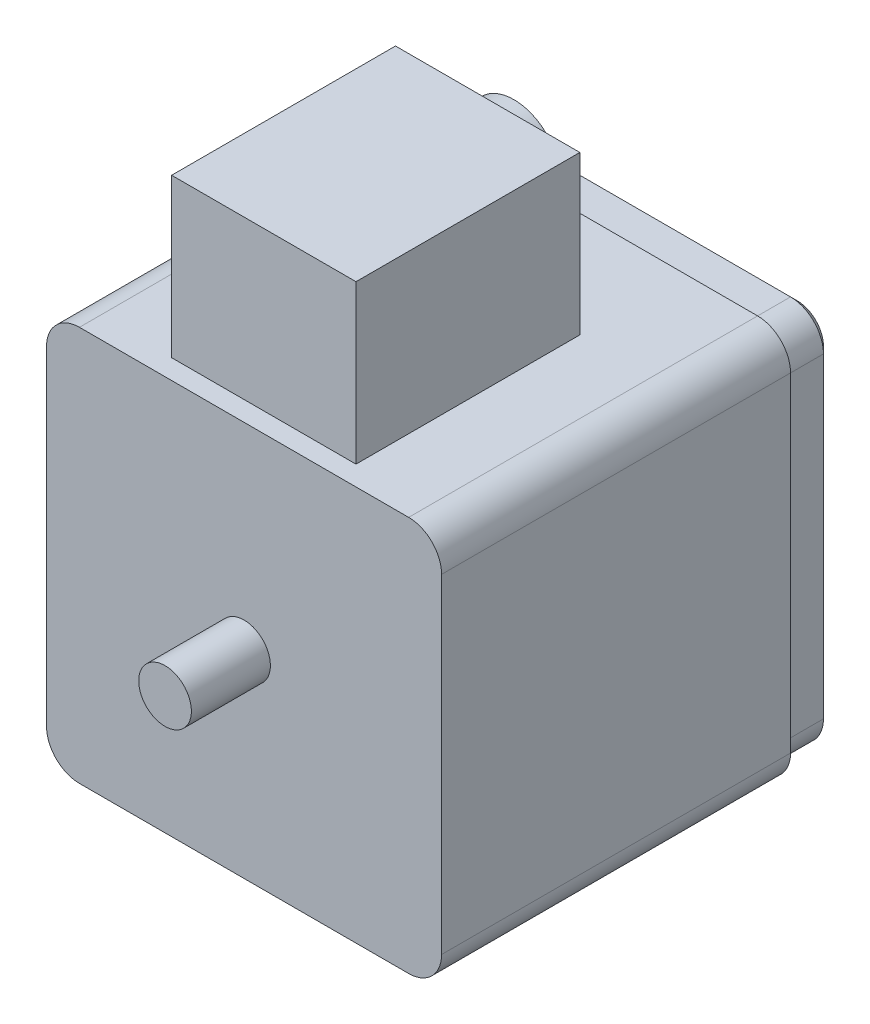
from build123d import *

# Parameters (mm, degrees)
SKETCH_1_W          = 60
SKETCH_1_H          = 60
EXTRUDE_1_DEPTH     = 60
SKETCH_3_R          = 4
EXTRUDE_2_DEPTH     = 12
SKETCH_4_W          = 60
SKETCH_4_H          = 60
SKETCH_4_W_2        = 58
SKETCH_4_H_2        = 58
CUT_EXTRUDE_4_DEPTH = 7
FILLET_4_R          = 5
CHAMFER_1_SIZE      = 1
FILLET_6_R          = 5
SKETCH_7_W          = 28
SKETCH_7_H          = 38
EXTRUDE_3_DEPTH     = 24
SKETCH_8_W          = 44.228024
SKETCH_8_H          = 29.89004
SKETCH_8_R          = 7
CUT_EXTRUDE_5_DEPTH = 4


with BuildPart() as part:
    # 草图1 → 凸台-拉伸1 (new body)
    with BuildSketch(Plane.XY):
        Rectangle(SKETCH_1_W, SKETCH_1_H)
    extrude(amount=EXTRUDE_1_DEPTH)

    # 草图3 → 凸台-拉伸2 (add)
    with BuildSketch(Plane.XY.offset(60)):
        Circle(SKETCH_3_R)
    extrude(amount=EXTRUDE_2_DEPTH)

    # 草图4 → 切除-拉伸4 (cut)
    with BuildSketch(Plane(origin=(0, 0, 0), x_dir=(-1, 0, 0), z_dir=(0, 0, -1))):
        Rectangle(SKETCH_4_W, SKETCH_4_H)
        Rectangle(SKETCH_4_W_2, SKETCH_4_H_2, mode=Mode.SUBTRACT)
    extrude(amount=-CUT_EXTRUDE_4_DEPTH, mode=Mode.SUBTRACT)

    # 圆角4
    fillet_4_edges = [part.edges().sort_by_distance(p)[0] for p in [
        (-29, -29, 3.5),
        (29, -29, 3.5),
        (29, 29, 3.5),
        (-29, 29, 3.5),
    ]]
    fillet(fillet_4_edges, radius=FILLET_4_R)

    # 倒角1
    chamfer_1_edges = [part.edges().sort_by_distance(p)[0] for p in [
        (0, 29, 0),
        (-29, 0, 0),
        (29, 0, 0),
        (0, -29, 0),
        (27.535533906, -27.535533906, 0),
        (-27.535533906, -27.535533906, 0),
        (-27.535533906, 27.535533906, 0),
        (27.535533906, 27.535533906, 0),
    ]]
    chamfer(chamfer_1_edges, length=CHAMFER_1_SIZE)

    # 圆角6
    fillet_6_edges = [part.edges().sort_by_distance(p)[0] for p in [
        (30, -30, 33.5),
        (-30, -30, 33.5),
        (-30, 30, 33.5),
        (30, 30, 33.5),
    ]]
    fillet(fillet_6_edges, radius=FILLET_6_R)

    # 草图7 → 凸台-拉伸3 (add)
    with BuildSketch(Plane(origin=(0, 30, 0), x_dir=(1, 0, 0), z_dir=(0, 1, 0))):
        with Locations((0, -38)):
            Rectangle(SKETCH_7_W, SKETCH_7_H)
    extrude(amount=EXTRUDE_3_DEPTH)

    # 草图8 → 切除-拉伸5 (cut)
    with BuildSketch(Plane(origin=(0, 0, 19), x_dir=(-1, 0, 0), z_dir=(0, 0, -1))):
        with Locations((0, 44.94502)):
            Rectangle(SKETCH_8_W, SKETCH_8_H)
        with Locations((0, 44.94502)):
            Circle(SKETCH_8_R, mode=Mode.SUBTRACT)
    extrude(amount=-CUT_EXTRUDE_5_DEPTH, mode=Mode.SUBTRACT)


solid = part.part
